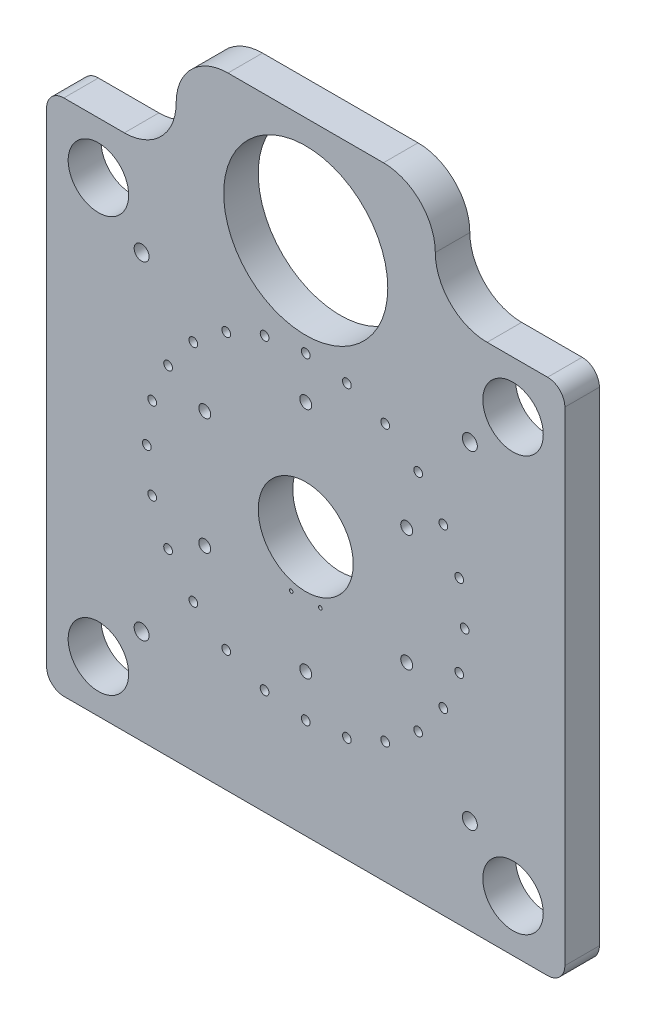
from build123d import *

# Parameters (mm, degrees)
SKETCH1_R                       = 49
SKETCH1_R_2                     = 55
SKETCH1_R_3                     = 5.053
SKETCH1_R_4                     = 95
SKETCH1_R_5                     = 6.9175
SKETCH1_R_6                     = 8.647
SKETCH1_R_7                     = 2.067
BOSS_EXTRUDE1_DEPTH             = 40
BOSS_EXTRUDE2_START             = -38
SKETCH2_R                       = 49
SKETCH2_R_2                     = 35
BOSS_EXTRUDE2_DEPTH             = 38
SIZE_MM_DOWEL_HOLE_1_AT_2_COUNT = 2
SIZE_MM_DOWEL_HOLE_1_AT_2_PITCH = 71.01408311
SIZE_MM_DOWEL_HOLE_1_AT_3_COUNT = 2
SIZE_MM_DOWEL_HOLE_1_AT_3_PITCH = 71.01408311
LPATTERN1_COUNT                 = 2
LPATTERN1_PITCH                 = 480
LPATTERN1_COUNT_DIR2            = 2
LPATTERN1_PITCH_DIR2            = 480


with BuildPart() as part:
    # Sketch1 → Boss-Extrude1 (new body)
    with BuildSketch(Plane.XY):
        with BuildLine():
            Line((-96.250646967, 420), (83.749353033, 420))
            ThreePointArc((83.749353033, 420), (126.175759905, 402.426406871), (143.749353033, 360))
            ThreePointArc((143.749353033, 360), (161.322946162, 317.573593129), (203.749353033, 300))
            Line((203.749353033, 300), (273.749353033, 300))
            ThreePointArc((273.749353033, 300), (287.891488657, 294.142135624), (293.749353033, 280))
            Line((293.749353033, 280), (293.749353033, -280))
            ThreePointArc((293.749353033, -280), (287.891488657, -294.142135624), (273.749353033, -300))
            Line((273.749353033, -300), (-286.250646967, -300))
            ThreePointArc((-286.250646967, -300), (-300.39278259, -294.142135624), (-306.250646967, -280))
            Line((-306.250646967, -280), (-306.250646967, 280))
            ThreePointArc((-306.250646967, 280), (-300.39278259, 294.142135624), (-286.250646967, 300))
            Line((-286.250646967, 300), (-216.250646967, 300))
            ThreePointArc((-216.250646967, 300), (-173.824240095, 317.573593129), (-156.250646967, 360))
            ThreePointArc((-156.250646967, 360), (-138.677053838, 402.426406871), (-96.250646967, 420))
        make_face()
        with Locations((-246.250646967, 240)):
            Circle(SKETCH1_R, mode=Mode.SUBTRACT)
        with Locations((233.749353033, -240)):
            Circle(SKETCH1_R, mode=Mode.SUBTRACT)
        with Locations((-246.250646967, -240)):
            Circle(SKETCH1_R, mode=Mode.SUBTRACT)
        with Locations((233.749353033, 240)):
            Circle(SKETCH1_R, mode=Mode.SUBTRACT)
        with Locations((-6.250646967, 0)):
            Circle(SKETCH1_R_2, mode=Mode.SUBTRACT)
        with Locations((-6.250646967, -184)):
            Circle(SKETCH1_R_3, mode=Mode.SUBTRACT)
        with Locations((-53.873351265, -177.730352037)):
            Circle(SKETCH1_R_3, mode=Mode.SUBTRACT)
        with Locations((-98.250646967, -159.348674296)):
            Circle(SKETCH1_R_3, mode=Mode.SUBTRACT)
        with Locations((-136.358294705, -130.107647738)):
            Circle(SKETCH1_R_3, mode=Mode.SUBTRACT)
        with Locations((-165.599321263, -92)):
            Circle(SKETCH1_R_3, mode=Mode.SUBTRACT)
        with Locations((-183.980999004, -47.622704299)):
            Circle(SKETCH1_R_3, mode=Mode.SUBTRACT)
        with Locations((-190.250646967, 0)):
            Circle(SKETCH1_R_3, mode=Mode.SUBTRACT)
        with Locations((-183.980999004, 47.622704299)):
            Circle(SKETCH1_R_3, mode=Mode.SUBTRACT)
        with Locations((-165.599321263, 92)):
            Circle(SKETCH1_R_3, mode=Mode.SUBTRACT)
        with Locations((-136.358294705, 130.107647738)):
            Circle(SKETCH1_R_3, mode=Mode.SUBTRACT)
        with Locations((-98.250646967, 159.348674296)):
            Circle(SKETCH1_R_3, mode=Mode.SUBTRACT)
        with Locations((-53.873351265, 177.730352037)):
            Circle(SKETCH1_R_3, mode=Mode.SUBTRACT)
        with Locations((-6.250646967, 184)):
            Circle(SKETCH1_R_3, mode=Mode.SUBTRACT)
        with Locations((41.372057332, 177.730352037)):
            Circle(SKETCH1_R_3, mode=Mode.SUBTRACT)
        with Locations((85.749353033, 159.348674296)):
            Circle(SKETCH1_R_3, mode=Mode.SUBTRACT)
        with Locations((123.857000772, 130.107647738)):
            Circle(SKETCH1_R_3, mode=Mode.SUBTRACT)
        with Locations((153.09802733, 92)):
            Circle(SKETCH1_R_3, mode=Mode.SUBTRACT)
        with Locations((171.479705071, 47.622704299)):
            Circle(SKETCH1_R_3, mode=Mode.SUBTRACT)
        with Locations((177.749353033, 0)):
            Circle(SKETCH1_R_3, mode=Mode.SUBTRACT)
        with Locations((171.479705071, -47.622704299)):
            Circle(SKETCH1_R_3, mode=Mode.SUBTRACT)
        with Locations((153.09802733, -92)):
            Circle(SKETCH1_R_3, mode=Mode.SUBTRACT)
        with Locations((123.857000772, -130.107647738)):
            Circle(SKETCH1_R_3, mode=Mode.SUBTRACT)
        with Locations((85.749353033, -159.348674296)):
            Circle(SKETCH1_R_3, mode=Mode.SUBTRACT)
        with Locations((41.372057332, -177.730352037)):
            Circle(SKETCH1_R_3, mode=Mode.SUBTRACT)
        with Locations((-6.250646967, 297)):
            Circle(SKETCH1_R_4, mode=Mode.SUBTRACT)
        with Locations((-6.250646967, 135)):
            Circle(SKETCH1_R_5, mode=Mode.SUBTRACT)
        with Locations((110.662782544, 67.5)):
            Circle(SKETCH1_R_5, mode=Mode.SUBTRACT)
        with Locations((110.662782544, -67.5)):
            Circle(SKETCH1_R_5, mode=Mode.SUBTRACT)
        with Locations((-6.250646967, -135)):
            Circle(SKETCH1_R_5, mode=Mode.SUBTRACT)
        with Locations((-123.164076477, -67.5)):
            Circle(SKETCH1_R_5, mode=Mode.SUBTRACT)
        with Locations((-123.164076477, 67.5)):
            Circle(SKETCH1_R_5, mode=Mode.SUBTRACT)
        with Locations((-196.250646967, 190)):
            Circle(SKETCH1_R_6, mode=Mode.SUBTRACT)
        with Locations((183.749353033, -190)):
            Circle(SKETCH1_R_6, mode=Mode.SUBTRACT)
        with Locations((-196.250646967, -190)):
            Circle(SKETCH1_R_6, mode=Mode.SUBTRACT)
        with Locations((183.749353033, 190)):
            Circle(SKETCH1_R_6, mode=Mode.SUBTRACT)
        with Locations((-23.073884898, -62.785178709)):
            Circle(SKETCH1_R_7, mode=Mode.SUBTRACT)
        with Locations((10.572590965, -62.785178709)):
            Circle(SKETCH1_R_7, mode=Mode.SUBTRACT)
    extrude(amount=BOSS_EXTRUDE1_DEPTH)

    # Sketch2 → Boss-Extrude2 (add)
    # profile 1 of 4: a face of its own
    with BuildSketch(Plane.XY.offset(40).offset(BOSS_EXTRUDE2_START)):
        with Locations((-246.250646967, 240)):
            Circle(SKETCH2_R)
        with Locations((-246.250646967, 240)):
            Circle(SKETCH2_R_2, mode=Mode.SUBTRACT)
    # profile 2 of 4: a face of its own
    with BuildSketch(Plane.XY.offset(40).offset(BOSS_EXTRUDE2_START)):
        with Locations((233.749353033, 240)):
            Circle(SKETCH2_R)
        with Locations((233.749353033, 240)):
            Circle(SKETCH2_R_2, mode=Mode.SUBTRACT)
    # profile 3 of 4: a face of its own
    with BuildSketch(Plane.XY.offset(40).offset(BOSS_EXTRUDE2_START)):
        with Locations((233.749353033, -240)):
            Circle(SKETCH2_R)
        with Locations((233.749353033, -240)):
            Circle(SKETCH2_R_2, mode=Mode.SUBTRACT)
    # profile 4 of 4: a face of its own
    with BuildSketch(Plane.XY.offset(40).offset(BOSS_EXTRUDE2_START)):
        with Locations((-246.250646967, -240)):
            Circle(SKETCH2_R)
        with Locations((-246.250646967, -240)):
            Circle(SKETCH2_R_2, mode=Mode.SUBTRACT)
    extrude(amount=BOSS_EXTRUDE2_DEPTH)

    # Sketch5 → Size mm Dowel hole 1 (revolve, cut)
    with BuildSketch(Plane(origin=(254.249353033, 275.507041555, 2), x_dir=(0, 1, 0), z_dir=(1, 0, 0))):
        Polygon((0, 0), (0, 12.76137699), (1.6, 11.8), (1.6, 0), align=None)
    size_mm_dowel_hole_1 = revolve(axis=Axis((254.249353033, 275.507041555, -4.35), (0, 0, 1)), mode=Mode.SUBTRACT)

    # Size mm Dowel hole 1 at 2: Size mm Dowel hole 1 ×2
    with Locations(*[Vector(-0.8660254037844366, -0.5000000000000037, 0) * (i * SIZE_MM_DOWEL_HOLE_1_AT_2_PITCH) for i in range(1, SIZE_MM_DOWEL_HOLE_1_AT_2_COUNT)]):
        add(size_mm_dowel_hole_1, mode=Mode.SUBTRACT)

    # Size mm Dowel hole 1 at 3: Size mm Dowel hole 1 ×2
    with Locations(*[(0, -i * SIZE_MM_DOWEL_HOLE_1_AT_3_PITCH, 0) for i in range(1, SIZE_MM_DOWEL_HOLE_1_AT_3_COUNT)]):
        add(size_mm_dowel_hole_1, mode=Mode.SUBTRACT)

    # LPattern1: Size mm Dowel hole 1 2 × 2
    with Locations(*[(-i * LPATTERN1_PITCH, -j * LPATTERN1_PITCH_DIR2, 0) for i in range(LPATTERN1_COUNT) for j in range(LPATTERN1_COUNT_DIR2) if (i, j) != (0, 0)]):
        add(size_mm_dowel_hole_1, mode=Mode.SUBTRACT)

    # LPattern1 copy 1 sketch → LPattern1 copy 1 (revolve, cut)
    with BuildSketch(Plane(origin=(192.749353033, -240, 2), x_dir=(0, 1, 0), z_dir=(1, 0, 0))):
        Polygon((0, 0), (0, 12.76137699), (1.6, 11.8), (1.6, 0), align=None)
    revolve(axis=Axis((192.749353033, -240, -4.35), (0, 0, 1)), mode=Mode.SUBTRACT)

    # LPattern1 copy 2 sketch → LPattern1 copy 2 (revolve, cut)
    with BuildSketch(Plane(origin=(-287.250646967, 240, 2), x_dir=(0, 1, 0), z_dir=(1, 0, 0))):
        Polygon((0, 0), (0, 12.76137699), (1.6, 11.8), (1.6, 0), align=None)
    revolve(axis=Axis((-287.250646967, 240, -4.35), (0, 0, 1)), mode=Mode.SUBTRACT)

    # LPattern1 copy 3 sketch → LPattern1 copy 3 (revolve, cut)
    with BuildSketch(Plane(origin=(-287.250646967, -240, 2), x_dir=(0, 1, 0), z_dir=(1, 0, 0))):
        Polygon((0, 0), (0, 12.76137699), (1.6, 11.8), (1.6, 0), align=None)
    revolve(axis=Axis((-287.250646967, -240, -4.35), (0, 0, 1)), mode=Mode.SUBTRACT)

    # LPattern1 copy 4 sketch → LPattern1 copy 4 (revolve, cut)
    with BuildSketch(Plane(origin=(254.249353033, -275.507041555, 2), x_dir=(0, 1, 0), z_dir=(1, 0, 0))):
        Polygon((0, 0), (0, 12.76137699), (1.6, 11.8), (1.6, 0), align=None)
    revolve(axis=Axis((254.249353033, -275.507041555, -4.35), (0, 0, 1)), mode=Mode.SUBTRACT)

    # LPattern1 copy 5 sketch → LPattern1 copy 5 (revolve, cut)
    with BuildSketch(Plane(origin=(-225.750646967, 204.492958445, 2), x_dir=(0, 1, 0), z_dir=(1, 0, 0))):
        Polygon((0, 0), (0, 12.76137699), (1.6, 11.8), (1.6, 0), align=None)
    revolve(axis=Axis((-225.750646967, 204.492958445, -4.35), (0, 0, 1)), mode=Mode.SUBTRACT)

    # LPattern1 copy 6 sketch → LPattern1 copy 6 (revolve, cut)
    with BuildSketch(Plane(origin=(-225.750646967, -275.507041555, 2), x_dir=(0, 1, 0), z_dir=(1, 0, 0))):
        Polygon((0, 0), (0, 12.76137699), (1.6, 11.8), (1.6, 0), align=None)
    revolve(axis=Axis((-225.750646967, -275.507041555, -4.35), (0, 0, 1)), mode=Mode.SUBTRACT)


solid = part.part
